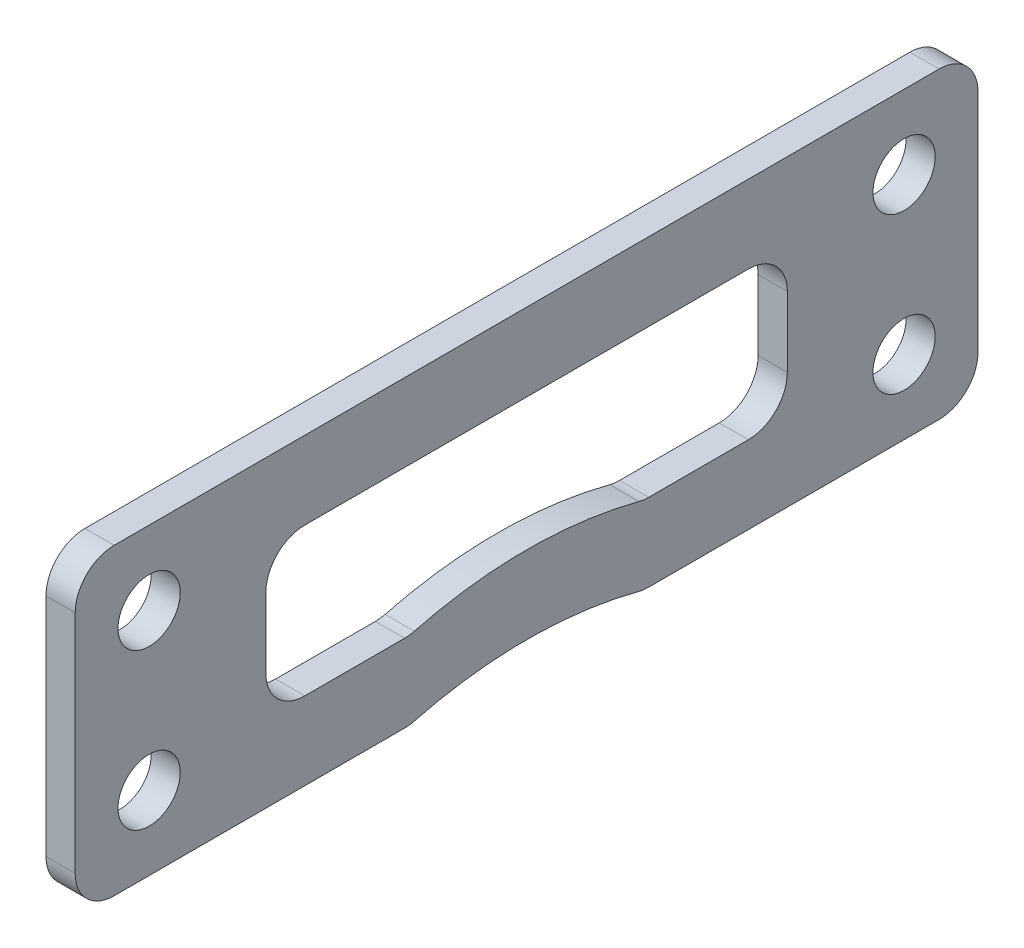
SolidWorks part; units mm, degrees
material "Thornel Mat VMA"
ref_plane "前视基准面" through (0, 0, 0) normal (0, 0, 1) x (1, 0, 0)
ref_plane "上视基准面" through (0, 0, 0) normal (0, 1, 0) x (1, 0, 0)
ref_plane "右视基准面" through (0, 0, 0) normal (1, 0, 0) x (0, 0, -1)
other "Configuration Table"
sketch "草图1" plane through (0, 0, 0) normal (1, 0, 0) x (0, 0, -1)
  line L0 (0, 0) -> (38.8, 0) construction
  line L2 (-3.8, 3.8) -> (42.6, 3.8)
  line L3 (-3.8, 3.8) -> (-3.8, -11.8)
  line L4 (-3.8, -11.8) -> (42.6, -11.8)
  line L5 (42.6, 3.8) -> (42.6, -11.8)
  circle A0 centre (0, 0) radius 1.6
  circle A1 centre (0, -8) radius 1.6
  circle A2 centre (38.8, 0) radius 1.6
  circle A3 centre (38.8, -8) radius 1.6
  dimension "D1" = 3.2
  dimension "D2" = 3.2
  dimension "D5" = 3.2
  dimension "D6" = 3.2
  dimension "D3" = 8
  dimension "D4" = 38.8
  dimension "D7" = 3.8
  dimension "D8" = 3.8
  dimension "D9" = 3.8
  dimension "D10" = 3.8
extrude "凸台-拉伸1" add sketch "草图1" along normal blind 1.5
sketch "草图2" plane through (1.5, 0, 0) normal (1, 0, 0) x (0, 0, -1)
  line L0 (38.8, -8) -> (19.4, -8) construction
  line L1 (19.4, -8) -> (19.4, -34) construction
  circle A0 centre (19.4, -34) radius 23
  dimension "D3" = 46
  dimension "D1" = 19.4
  dimension "D2" = 26
extrude "切除-拉伸1" cut sketch "草图2" against normal through all
sketch "草图3" plane through (1.5, 0, 0) normal (1, 0, 0) x (0, 0, -1)
  line L0 (42.6, 3.8) -> (-3.8, 3.8) construction
  line L1 (6, -0.2) -> (32.8, -0.2)
  line L2 (6, -0.2) -> (6, -7.8)
  line L3 (6, -7.8) -> (13.3867, -7.8)
  line L4 (32.8, -0.2) -> (32.8, -7.8)
  line L5 (-3.8, -11.8) -> (13.3867, -11.8) construction
  line L6 (19.4, -34) -> (19.4, -30) construction
  line L7 (25.4133, -7.8) -> (32.8, -7.8)
  circle A0 centre (0, 0) radius 1.6 construction
  circle A1 centre (38.8, 0) radius 1.6 construction
  arc A2 (25.4133, -7.8) -> (13.3867, -7.8) centre (19.4, -30) ccw
  dimension "D5" = 46
  dimension "D1" = 6
  dimension "D2" = 6
  dimension "D3" = 4
  dimension "D4" = 4
  dimension "D6" = 4
extrude "切除-拉伸2" cut sketch "草图3" against normal through all
fillet "圆角1" radius 2 12 edges at (0.75, -11.8, -42.6) (0.75, 3.8, -42.6) (0.75, 3.8, 3.8) (0.75, -11.8, 3.8) (0.75, -11.8, -25.4133) (0.75, -11.8, -13.3867) (0.75, -0.2, -32.8) (0.75, -7.8, -32.8) (0.75, -7.8, -25.4133) (0.75, -7.8, -13.3867) (0.75, -7.8, -6) (0.75, -0.2, -6)
